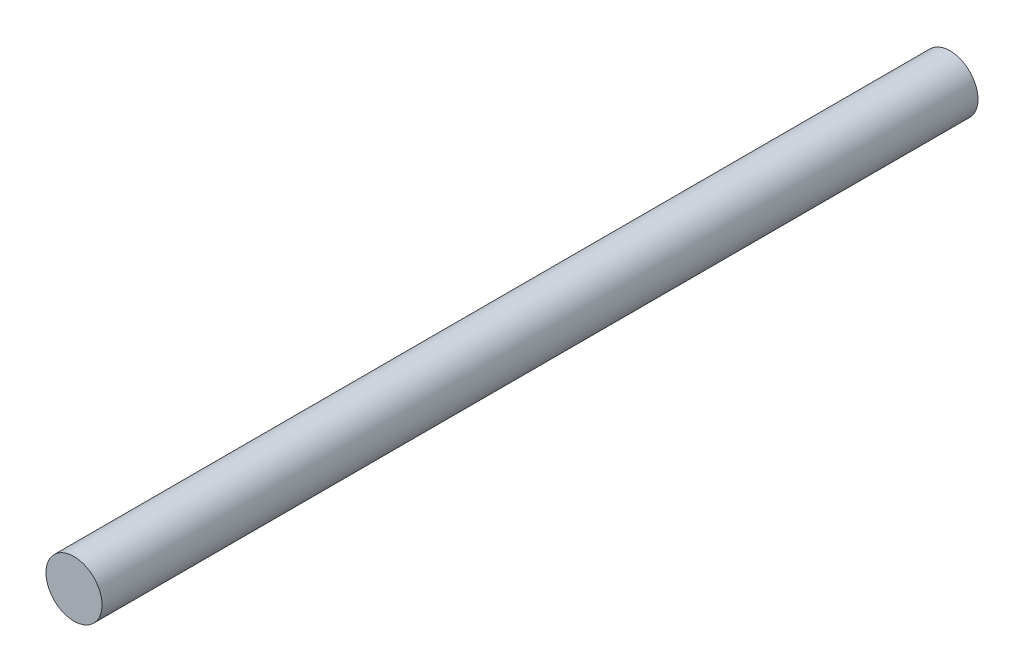
from build123d import *

# Parameters (mm, degrees)
SKETCH_1_R      = 8
EXTRUDE_1_DEPTH = 250


with BuildPart() as part:
    # 草图1 → 凸台-拉伸1 (new body)
    with BuildSketch(Plane.XY):
        Circle(SKETCH_1_R)
    extrude(amount=EXTRUDE_1_DEPTH)


solid = part.part
